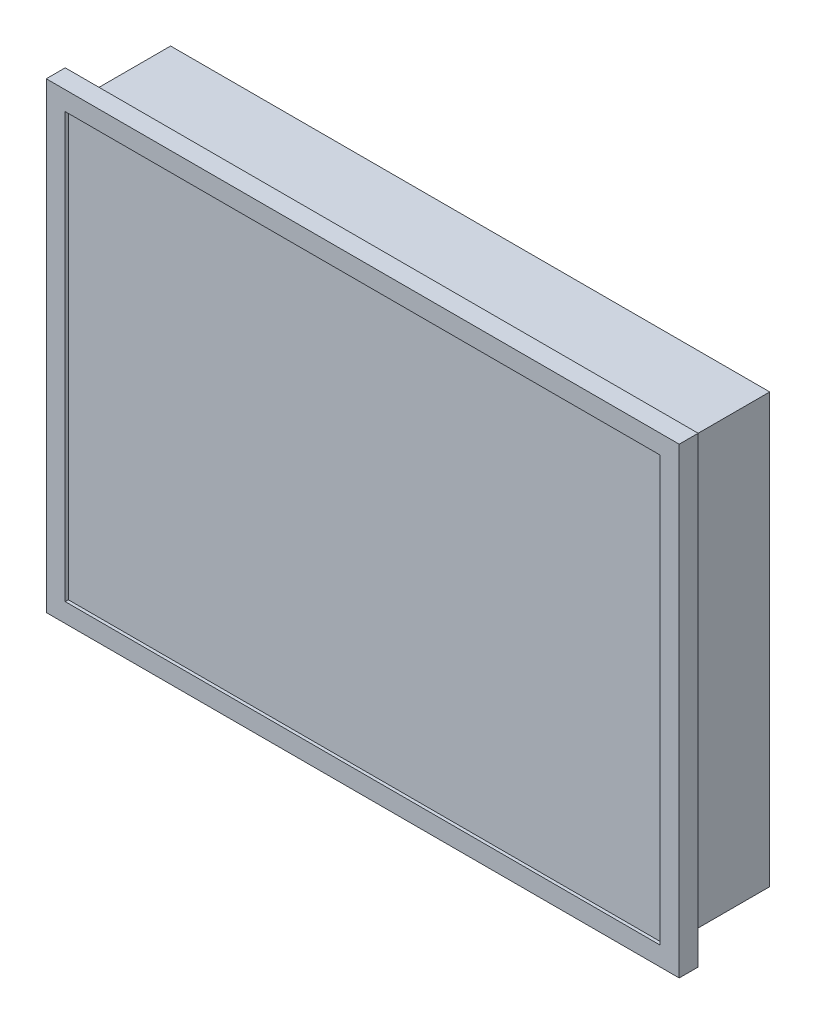
SolidWorks part; units mm, degrees
material "A6061"
ref_plane "前视基准面" through (0, 0, 0) normal (0, 0, 1) x (1, 0, 0)
ref_plane "上视基准面" through (0, 0, 0) normal (0, 1, 0) x (1, 0, 0)
ref_plane "右视基准面" through (0, 0, 0) normal (1, 0, 0) x (0, 0, -1)
sketch "草图1" plane through (0, 0, 0) normal (0, 0, 1) x (1, 0, 0)
  line L1 (-100.15, 73.15) -> (100.15, 73.15)
  line L2 (-100.15, 73.15) -> (-100.15, -73.15)
  line L3 (-100.15, -73.15) -> (100.15, -73.15)
  line L4 (100.15, 73.15) -> (100.15, -73.15)
  line L5 (-100.15, 73.15) -> (100.15, -73.15) construction
  line L6 (-100.15, -73.15) -> (100.15, 73.15) construction
  point P0 (0, 0)
  dimension "D1" = 200.3
  dimension "D2" = 146.3
extrude "凸台-拉伸1" add sketch "草图1" along normal blind 6
sketch "草图2" plane through (0, 0, 0) normal (0, 0, -1) x (-1, 0, 0)
  line L1 (-94.8, 67.8) -> (94.8, 67.8)
  line L2 (-94.8, 67.8) -> (-94.8, -67.8)
  line L3 (-94.8, -67.8) -> (94.8, -67.8)
  line L4 (94.8, 67.8) -> (94.8, -67.8)
  line L5 (-94.8, 67.8) -> (94.8, -67.8) construction
  line L6 (-94.8, -67.8) -> (94.8, 67.8) construction
  point P0 (0, 0)
  dimension "D1" = 189.6
  dimension "D2" = 135.6
extrude "凸台-拉伸2" add sketch "草图2" along normal blind 28
sketch "草图3" plane through (0, 0, 6) normal (0, 0, 1) x (1, 0, 0)
  line L0 (100.15, -73.15) -> (100.15, 73.15) construction
  line L1 (-94.15, 67.15) -> (94.15, 67.15)
  line L2 (-94.15, 67.15) -> (-94.15, -67.15)
  line L3 (-94.15, -67.15) -> (94.15, -67.15)
  line L4 (94.15, 67.15) -> (94.15, -67.15)
  line L5 (-94.15, 67.15) -> (94.15, -67.15) construction
  line L6 (-94.15, -67.15) -> (94.15, 67.15) construction
  line L7 (100.15, 73.15) -> (-100.15, 73.15) construction
  point P0 (0, 0)
  dimension "D1" = 6
  dimension "D2" = 6
extrude "切除-拉伸1" cut sketch "草图3" against normal blind 1
